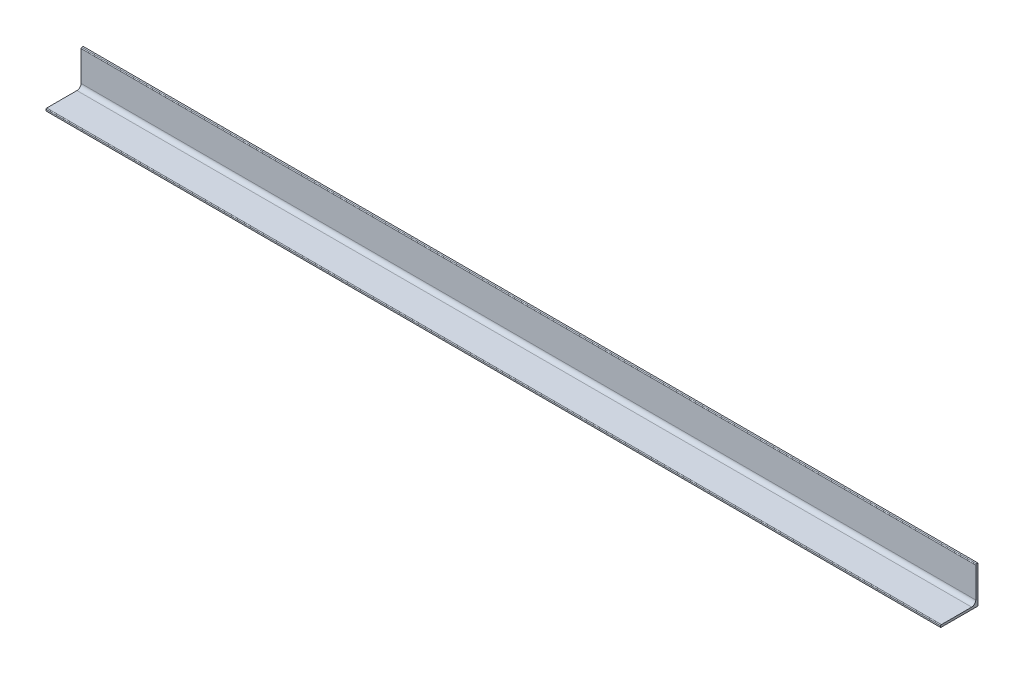
from build123d import *

# Parameters (mm, degrees)
BASE_DEPTH = 1200


with BuildPart() as part:
    # Sketch1 → Base (new body)
    with BuildSketch(Plane.YZ):
        with BuildLine():
            Line((0, 50), (0, 0))
            Line((0, 0), (50, 0))
            Line((50, 0), (50, 2))
            ThreePointArc((50, 2), (49.707106781, 2.707106781), (49, 3))
            Line((49, 3), (8.5, 3))
            ThreePointArc((8.5, 3), (4.610912703, 4.610912703), (3, 8.5))
            Line((3, 8.5), (3, 49))
            ThreePointArc((3, 49), (2.707106781, 49.707106781), (2, 50))
            Line((2, 50), (0, 50))
        make_face()
    extrude(amount=BASE_DEPTH)


solid = part.part
